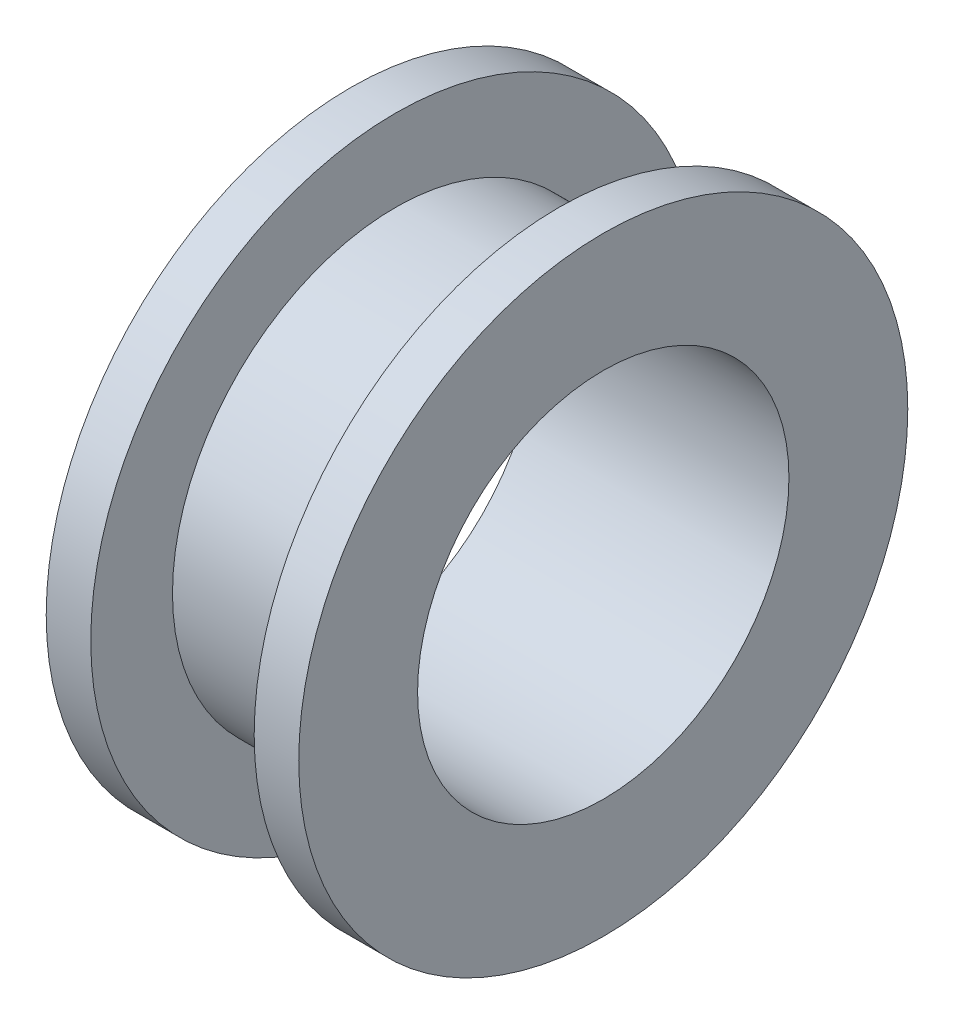
from build123d import *


with BuildPart() as part:
    # 草图1 → 旋转1 (revolve)
    with BuildSketch(Plane.XY, mode=Mode.PRIVATE) as revolve_1_sk:
        Polygon((0, 25), (0, 41), (6, 41), (6, 30), (28, 30), (28, 41), (34, 41), (34, 25), align=None)
    revolve(revolve_1_sk.sketch.rotate(Axis((0, 0, 0), (1, 0, 0)), 90), axis=Axis((0, 0, 0), (1, 0, 0)))


solid = part.part
